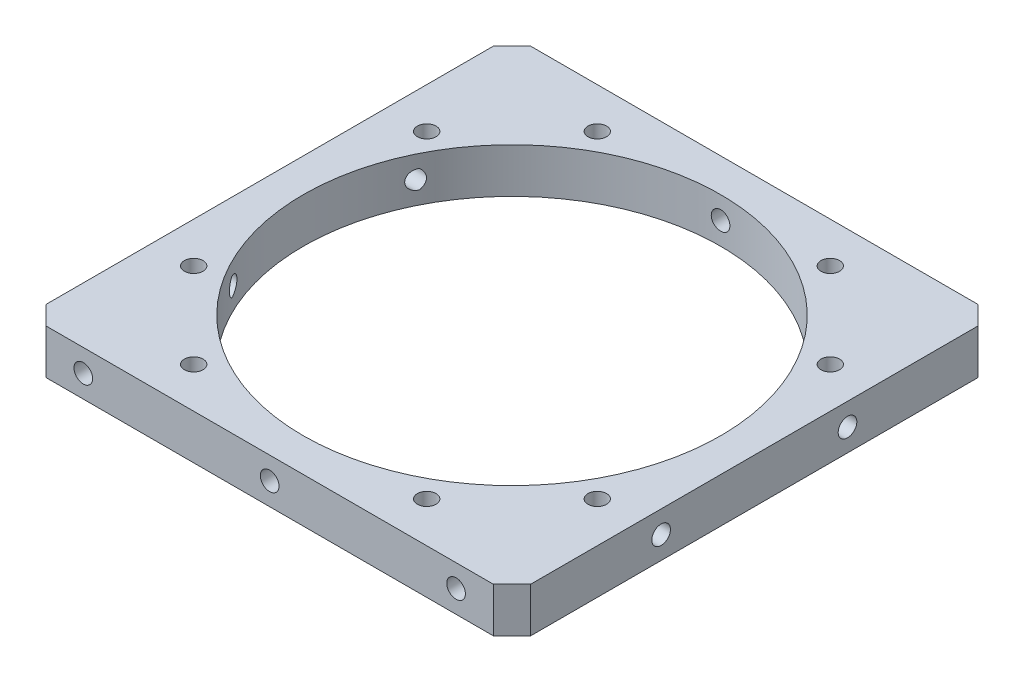
from build123d import *

# Parameters (mm, degrees)
SKETCH_1_W             = 130
SKETCH_1_H             = 130
EXTRUDE_1_DEPTH        = 12
SKETCH_2_R             = 56
CUT_EXTRUDE_1_DEPTH    = 93.703829479
HOLE_WIZARD_M6_1_D     = 5
HOLE_WIZARD_M6_2_D     = 5
HOLE_WIZARD_M6_2_DEPTH = 15
HOLE_WIZARD_M6_2_TIP   = 1.502151548
HOLE_WIZARD_M6_3_D     = 5
HOLE_WIZARD_M6_3_DEPTH = 15
HOLE_WIZARD_M6_3_TIP   = 1.502151548
HOLE_WIZARD_M6_4_D     = 5
HOLE_WIZARD_M6_4_DEPTH = 15
HOLE_WIZARD_M6_4_TIP   = 1.502151548
HOLE_WIZARD_M6_5_D     = 5
HOLE_WIZARD_M6_5_DEPTH = 15
HOLE_WIZARD_M6_5_TIP   = 1.502151548
CHAMFER_1_SIZE         = 5


with BuildPart() as part:
    # 草图1 → 凸台-拉伸1 (new body)
    with BuildSketch(Plane(origin=(0, 0, 0), x_dir=(1, 0, 0), z_dir=(0, 1, 0))):
        Rectangle(SKETCH_1_W, SKETCH_1_H)
    extrude(amount=EXTRUDE_1_DEPTH)

    # 草图2 → 切除-拉伸1 (cut, through all)
    with BuildSketch(Plane(origin=(0, 12, 0), x_dir=(1, 0, 0), z_dir=(0, 1, 0))):
        with Locations(Location((0, 0, 0), (0, 0, 270))):
            Circle(SKETCH_2_R)
    extrude(amount=-CUT_EXTRUDE_1_DEPTH, mode=Mode.SUBTRACT)

    # M6 螺纹孔1 (through all)
    with Locations(Plane(origin=(0, 12, 0), x_dir=(1, 0, 0), z_dir=(0, 1, 0))):
        with Locations((31.250000582, 54.1265874), (54.126588073, 31.249999418), (54.1265874, -31.250000582), (31.249999418, -54.126588073), (-31.250000582, -54.1265874), (-54.126588073, -31.249999418), (-54.1265874, 31.250000582), (-31.249999418, 54.126588073)):
            Hole(HOLE_WIZARD_M6_1_D / 2)

    # M6 螺纹孔2
    with Locations(Plane(origin=(65, 0, 0), x_dir=(0, 0, -1), z_dir=(1, 0, 0))):
        with Locations((-25, 6), (25, 6)):
            Hole(HOLE_WIZARD_M6_2_D / 2, depth=HOLE_WIZARD_M6_2_DEPTH)
            with Locations((0, 0, -(HOLE_WIZARD_M6_2_DEPTH + HOLE_WIZARD_M6_2_TIP / 2))):  # 118° drill point
                Cone(0, HOLE_WIZARD_M6_2_D / 2, HOLE_WIZARD_M6_2_TIP, mode=Mode.SUBTRACT)

    # M6 螺纹孔3
    with Locations(Plane.ZY.offset(65)):
        with Locations((-25, 6), (25, 6)):
            Hole(HOLE_WIZARD_M6_3_D / 2, depth=HOLE_WIZARD_M6_3_DEPTH)
            with Locations((0, 0, -(HOLE_WIZARD_M6_3_DEPTH + HOLE_WIZARD_M6_3_TIP / 2))):  # 118° drill point
                Cone(0, HOLE_WIZARD_M6_3_D / 2, HOLE_WIZARD_M6_3_TIP, mode=Mode.SUBTRACT)

    # M6 螺纹孔4
    with Locations(Plane(origin=(0, 0, -65), x_dir=(-1, 0, 0), z_dir=(0, 0, -1))):
        with Locations((-50, 6), (50, 6), (0, 6)):
            Hole(HOLE_WIZARD_M6_4_D / 2, depth=HOLE_WIZARD_M6_4_DEPTH)
            with Locations((0, 0, -(HOLE_WIZARD_M6_4_DEPTH + HOLE_WIZARD_M6_4_TIP / 2))):  # 118° drill point
                Cone(0, HOLE_WIZARD_M6_4_D / 2, HOLE_WIZARD_M6_4_TIP, mode=Mode.SUBTRACT)

    # M6 螺纹孔5
    with Locations(Plane.XY.offset(65)):
        with Locations((-50, 6), (50, 6), (0, 6)):
            Hole(HOLE_WIZARD_M6_5_D / 2, depth=HOLE_WIZARD_M6_5_DEPTH)
            with Locations((0, 0, -(HOLE_WIZARD_M6_5_DEPTH + HOLE_WIZARD_M6_5_TIP / 2))):  # 118° drill point
                Cone(0, HOLE_WIZARD_M6_5_D / 2, HOLE_WIZARD_M6_5_TIP, mode=Mode.SUBTRACT)

    # 倒角1
    chamfer_1_edges = [part.edges().sort_by_distance(p)[0] for p in [
        (65, 6, 65),
        (-65, 6, 65),
        (-65, 6, -65),
        (65, 6, -65),
    ]]
    chamfer(chamfer_1_edges, length=CHAMFER_1_SIZE)


solid = part.part
